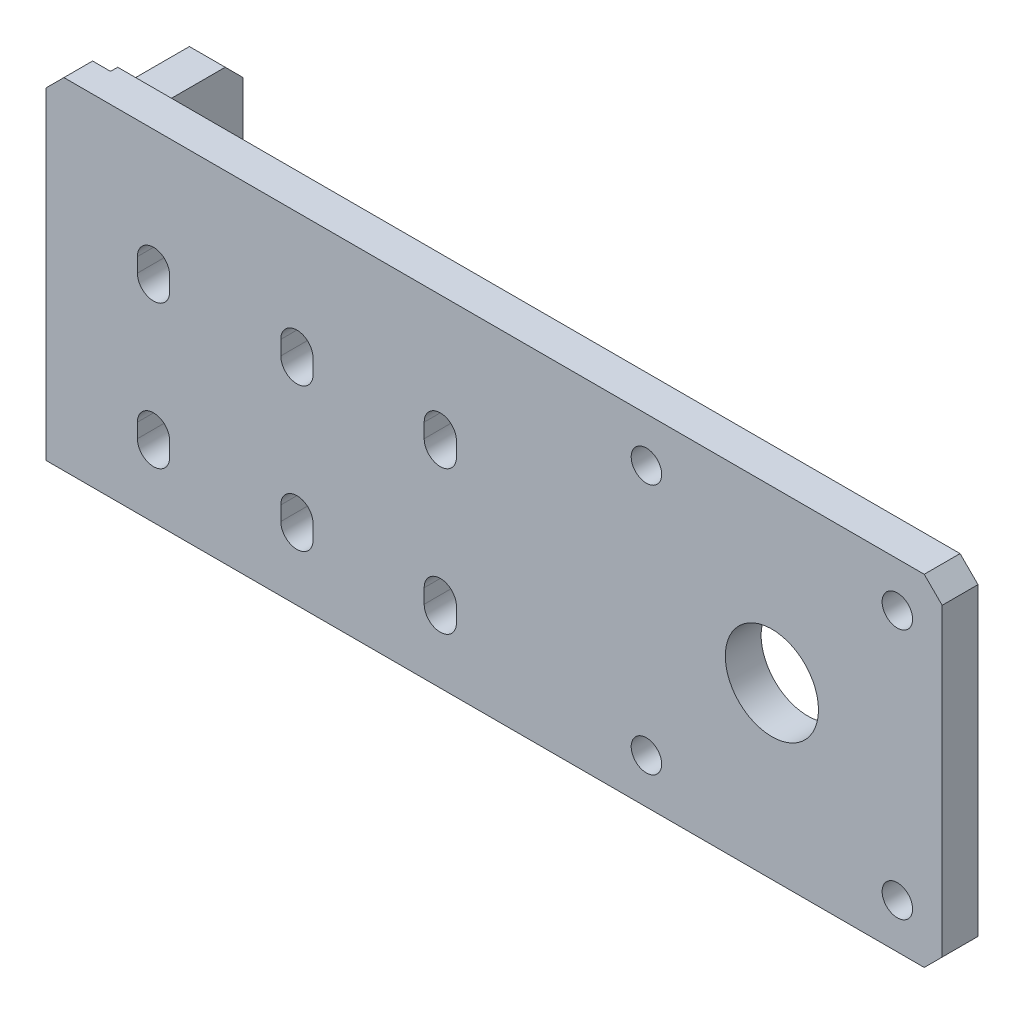
from build123d import *

# Parameters (mm, degrees)
SKETCH_1_W                  = 250
SKETCH_1_H                  = 95
EXTRUDE_1_DEPTH             = 10
CUT_EXTRUDE_2_DEPTH         = 135.094183319
PATTERN_LINEAR_1_COUNT      = 2
PATTERN_LINEAR_1_PITCH      = 40
PATTERN_LINEAR_1_COUNT_DIR2 = 2
PATTERN_LINEAR_1_PITCH_DIR2 = 40
PATTERN_LINEAR_2_COUNT      = 2
PATTERN_LINEAR_2_PITCH      = 40
PATTERN_LINEAR_2_COUNT_DIR2 = 2
PATTERN_LINEAR_2_PITCH_DIR2 = 40
HOLE_WIZARD_M10_3_D         = 8.5
HOLE_WIZARD_M10_3_DEPTH     = 24.5
HOLE_WIZARD_M10_3_TIP       = 2.553657631
SKETCH_12_R                 = 13
CUT_EXTRUDE_5_DEPTH         = 135.094183319
HOLE_WIZARD_M4_1_D          = 3.3
HOLE_WIZARD_M4_1_DEPTH      = 10.1
HOLE_WIZARD_M4_1_TIP        = 0.991420021
SKETCH_22_W                 = 10
SKETCH_22_H                 = 95
CUT_EXTRUDE_6_DEPTH         = 2
SKETCH_21_W                 = 10
SKETCH_21_H                 = 80
EXTRUDE_2_DEPTH             = 37
CHAMFER_1_SIZE              = 5
CHAMFER_2_SIZE              = 5


with BuildPart() as part:
    # 草图1 → 凸台-拉伸1 (new body)
    with BuildSketch(Plane.XY):
        Rectangle(SKETCH_1_W, SKETCH_1_H)
    extrude(amount=EXTRUDE_1_DEPTH)

    # 草图3 → 切除-拉伸2 (cut, through all)
    with BuildSketch(Plane.XY.offset(10)):
        with BuildLine():
            Line((-59.5, -29.5), (-59.5, -25.5))
            ThreePointArc((-59.5, -25.5), (-55, -21), (-50.5, -25.5))
            Line((-50.5, -25.5), (-50.5, -29.5))
            ThreePointArc((-50.5, -29.5), (-55, -34), (-59.5, -29.5))
        make_face()
    cut_extrude_2 = extrude(amount=-CUT_EXTRUDE_2_DEPTH, mode=Mode.SUBTRACT)

    # 阵列(线性)1: Cut-Extrude 2 2 × 2
    with Locations(*[(i * PATTERN_LINEAR_1_PITCH, j * PATTERN_LINEAR_1_PITCH_DIR2, 0) for i in range(PATTERN_LINEAR_1_COUNT) for j in range(PATTERN_LINEAR_1_COUNT_DIR2) if (i, j) != (0, 0)]):
        add(cut_extrude_2, mode=Mode.SUBTRACT)

    # 阵列(线性)2: Cut-Extrude 2 2 × 2
    with Locations(*[(-i * PATTERN_LINEAR_2_PITCH, j * PATTERN_LINEAR_2_PITCH_DIR2, 0) for i in range(PATTERN_LINEAR_2_COUNT) for j in range(PATTERN_LINEAR_2_COUNT_DIR2) if (i, j) != (0, 0)]):
        add(cut_extrude_2, mode=Mode.SUBTRACT)

    # M10 螺纹孔3
    with Locations(Plane(origin=(42.5, 35, 10), x_dir=(1, 0, 0), z_dir=(0, 0, 1))):
        with Locations((0, 0), (70, 0), (70, -70), (0, -70)):
            Hole(HOLE_WIZARD_M10_3_D / 2, depth=HOLE_WIZARD_M10_3_DEPTH)
            with Locations((0, 0, -(HOLE_WIZARD_M10_3_DEPTH + HOLE_WIZARD_M10_3_TIP / 2))):  # 118° drill point
                Cone(0, HOLE_WIZARD_M10_3_D / 2, HOLE_WIZARD_M10_3_TIP, mode=Mode.SUBTRACT)

    # 草图12 → 切除-拉伸5 (cut, through all)
    with BuildSketch(Plane.XY.offset(10)):
        with Locations((77.5, 0)):
            Circle(SKETCH_12_R)
    extrude(amount=-CUT_EXTRUDE_5_DEPTH, mode=Mode.SUBTRACT)

    # M4 螺纹孔1
    with Locations(Plane(origin=(117, -47.5, 5), x_dir=(0, 0, -1), z_dir=(0, -1, 0))):
        with Locations((0, 0), (0, -105), (0, -52.5)):
            Hole(HOLE_WIZARD_M4_1_D / 2, depth=HOLE_WIZARD_M4_1_DEPTH)
            with Locations((0, 0, -(HOLE_WIZARD_M4_1_DEPTH + HOLE_WIZARD_M4_1_TIP / 2))):  # 118° drill point
                Cone(0, HOLE_WIZARD_M4_1_D / 2, HOLE_WIZARD_M4_1_TIP, mode=Mode.SUBTRACT)

    # 草图22 → 切除-拉伸6 (cut)
    with BuildSketch(Plane(origin=(0, 0, 0), x_dir=(-1, 0, 0), z_dir=(0, 0, -1))):
        with Locations((120, 0)):
            Rectangle(SKETCH_22_W, SKETCH_22_H)
    extrude(amount=-CUT_EXTRUDE_6_DEPTH, mode=Mode.SUBTRACT)

    # 倒角1
    chamfer_1_edges = [part.edges().sort_by_distance(p)[0] for p in [
        (125, -47.5, 5),
        (-125, 47.5, 6),
        (125, 47.5, 5),
    ]]
    chamfer(chamfer_1_edges, length=CHAMFER_1_SIZE)


with BuildPart() as body_2:
    # 草图21 → 凸台-拉伸2 (new body)
    with BuildSketch(Plane(origin=(0, 0, 2), x_dir=(-1, 0, 0), z_dir=(0, 0, -1))):
        with Locations((120, -7.5)):
            Rectangle(SKETCH_21_W, SKETCH_21_H)
    extrude(amount=EXTRUDE_2_DEPTH)

    # 倒角2
    chamfer_2_edges = [body_2.edges().sort_by_distance(p)[0] for p in [
        (-120, -47.5, -35),
        (-120, 32.5, -35),
    ]]
    chamfer(chamfer_2_edges, length=CHAMFER_2_SIZE)


solid = Compound([part.part, body_2.part])
